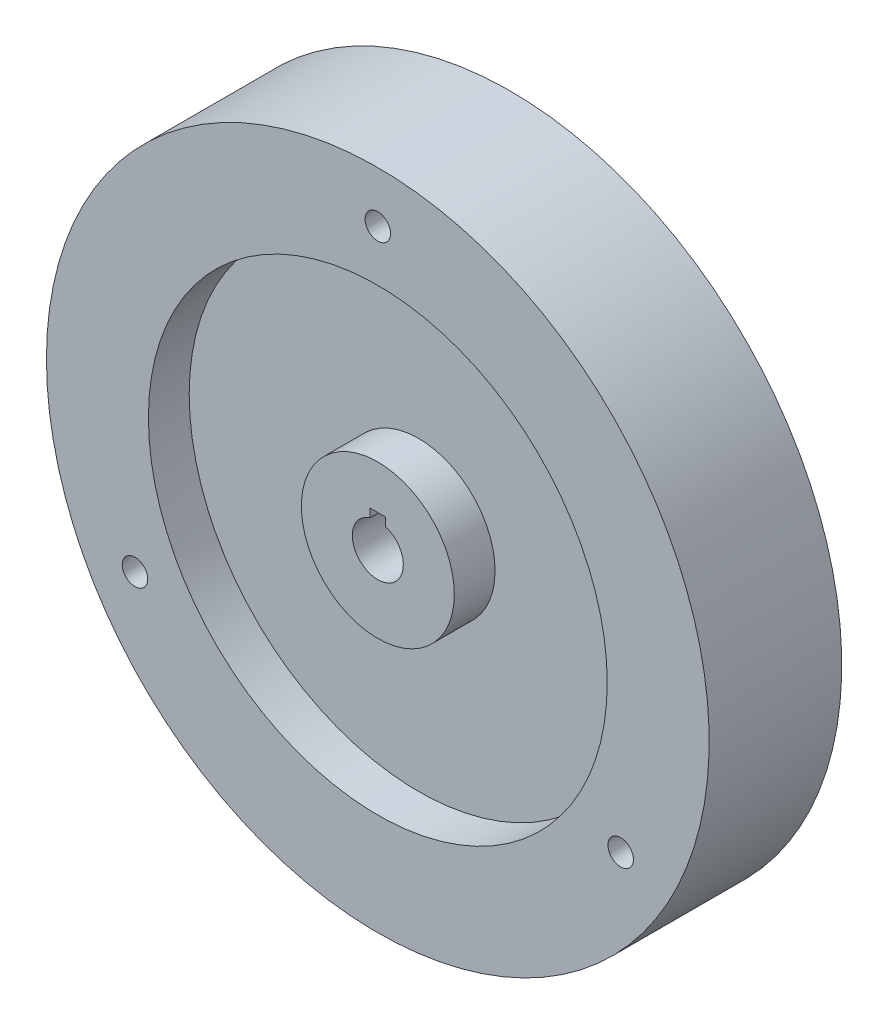
SolidWorks part; units mm, degrees
ref_plane "Front Plane" through (0, 0, 0) normal (0, 0, 1) x (1, 0, 0)
ref_plane "Top Plane" through (0, 0, 0) normal (0, 1, 0) x (1, 0, 0)
ref_plane "Right Plane" through (0, 0, 0) normal (1, 0, 0) x (0, 0, -1)
sketch "Sketch1" plane through (0, 0, 0) normal (0, 0, 1) x (1, 0, 0)
  circle A0 centre (0, 0) radius 65
  circle A1 centre (0, 0) radius 55 construction
  circle A2 centre (0, 55) radius 2.5
  circle A3 centre (47.6314, -27.5) radius 2.5
  circle A4 centre (-47.6314, -27.5) radius 2.5
  point P13 (0, 0)
  dimension "D1" = 130
  dimension "D2" = 110
  dimension "D3" = 5
  dimension "D4" = 3
extrude "Boss-Extrude1" add sketch "Sketch1" along normal blind 26
sketch "Sketch2" plane through (0, 0, 26) normal (0, 0, 1) x (1, 0, 0)
  line L1 (-1.5, 6.4034) -> (1.5, 6.4034)
  line L2 (-1.5, 6.4034) -> (-1.5, 4.7697)
  line L4 (1.5, 6.4034) -> (1.5, 4.7697)
  line L5 (-1.5, 6.4034) -> (0, 5) construction
  line L6 (0, 5) -> (1.5, 6.4034) construction
  arc A0 (-1.5, 4.7697) -> (1.5, 4.7697) centre (0, 0) ccw
  point P2 (0, 5)
  dimension "D1" = 10
extrude "Cut-Extrude1" cut sketch "Sketch2" against normal through all
sketch "Sketch3" plane through (0, 0, 26) normal (0, 0, 1) x (1, 0, 0)
  circle A0 centre (0, 0) radius 15
  circle A1 centre (0, 0) radius 45
  dimension "D1" = 90
  dimension "D2" = 30
extrude "Cut-Extrude2" cut sketch "Sketch3" against normal blind 8
sketch "Sketch4" plane through (0, 0, 0) normal (0, 0, -1) x (-1, 0, 0)
  circle A0 centre (0, 0) radius 15
  circle A1 centre (0, 0) radius 45
  dimension "D1" = 90
  dimension "D2" = 30
extrude "Cut-Extrude3" cut sketch "Sketch4" against normal blind 8
